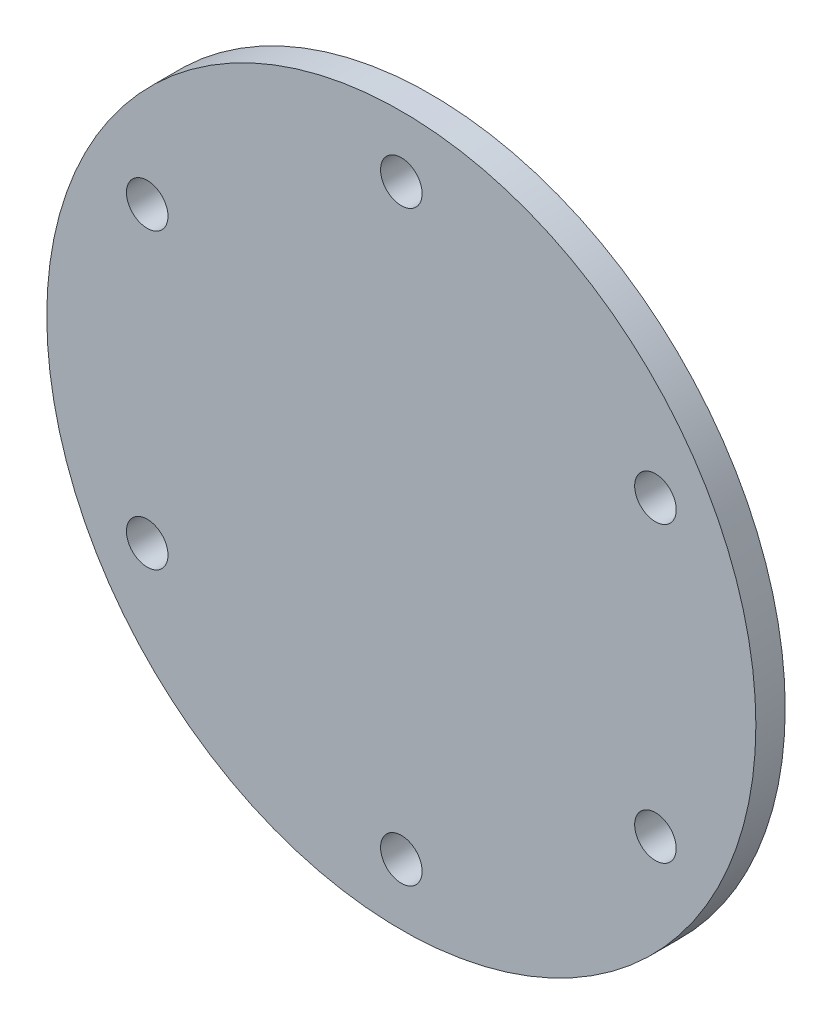
from build123d import *

# Parameters (mm, degrees)
SKETCH1_R           = 72.5
SKETCH1_R_2         = 4.25
BOSS_EXTRUDE1_DEPTH = 6


with BuildPart() as part:
    # Sketch1 → Boss-Extrude1 (new body)
    with BuildSketch(Plane.XY):
        Circle(SKETCH1_R)
        with Locations((0, 60)):
            Circle(SKETCH1_R_2, mode=Mode.SUBTRACT)
        with Locations((51.961524227, 30)):
            Circle(SKETCH1_R_2, mode=Mode.SUBTRACT)
        with Locations((51.961524227, -30)):
            Circle(SKETCH1_R_2, mode=Mode.SUBTRACT)
        with Locations((0, -60)):
            Circle(SKETCH1_R_2, mode=Mode.SUBTRACT)
        with Locations((-51.961524227, -30)):
            Circle(SKETCH1_R_2, mode=Mode.SUBTRACT)
        with Locations((-51.961524227, 30)):
            Circle(SKETCH1_R_2, mode=Mode.SUBTRACT)
    extrude(amount=BOSS_EXTRUDE1_DEPTH)


solid = part.part
